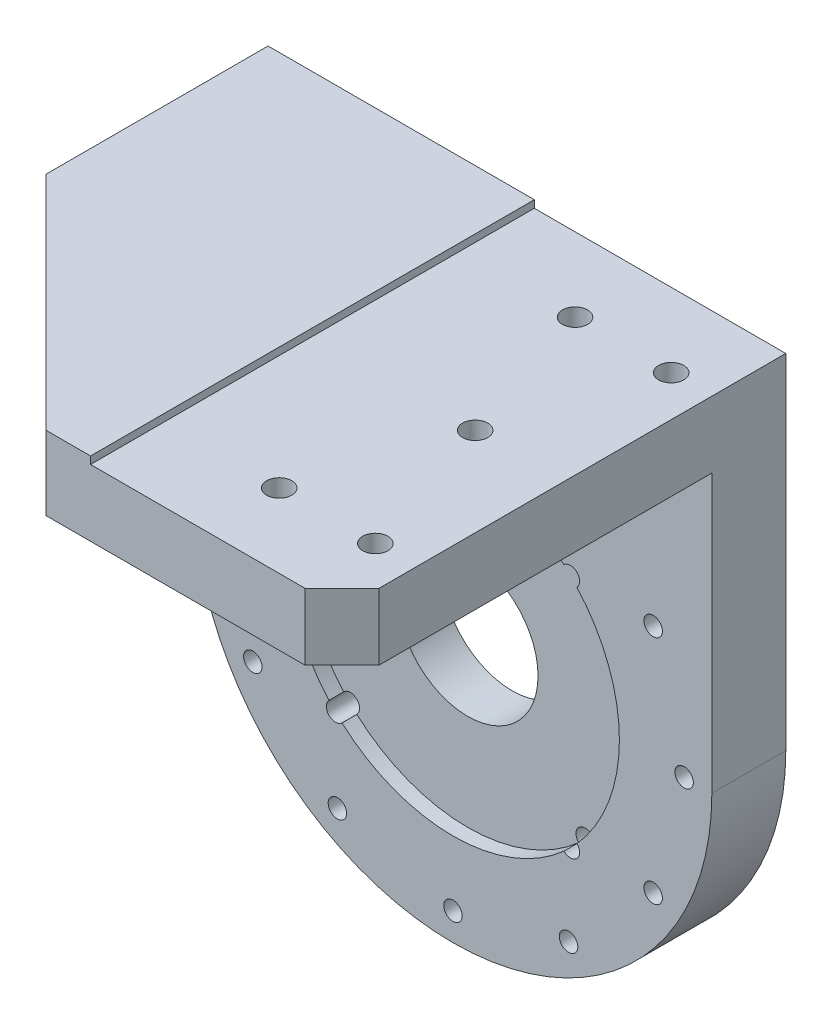
from build123d import *

# Parameters (mm, degrees)
EXTRUDE_1_DEPTH        = 20
SKETCH_2_R             = 45
CUT_EXTRUDE_1_DEPTH    = 4
SKETCH_3_R             = 19
CUT_EXTRUDE_2_DEPTH    = 104.831594421
SKETCH_4_R             = 35
CUT_EXTRUDE_3_DEPTH    = 4
HOLE_WIZARD_M6_1_D     = 5
HOLE_WIZARD_M6_2_D     = 5
SKETCH_15_W            = 140
SKETCH_15_H            = 120
EXTRUDE_2_DEPTH        = 20
SKETCH_20_W            = 68
SKETCH_20_H            = 120
CUT_EXTRUDE_4_DEPTH    = 2
CHAMFER_1_SIZE         = 10
CHAMFER_2_SIZE         = 60
HOLE_WIZARD_M8_1_D     = 6.8
HOLE_WIZARD_M8_1_DEPTH = 20


with BuildPart() as part:
    # 草图1 → 凸台-拉伸1 (new body)
    with BuildSketch(Plane.XY):
        with BuildLine():
            Line((-70, 0), (-70, 75))
            Line((-70, 75), (70, 75))
            Line((70, 75), (70, 0))
            ThreePointArc((70, 0), (0, -70), (-70, 0))
        make_face()
    extrude(amount=EXTRUDE_1_DEPTH)

    # 草图2 → 切除-拉伸1 (cut)
    with BuildSketch(Plane.XY.offset(20)):
        Circle(SKETCH_2_R)
    extrude(amount=-CUT_EXTRUDE_1_DEPTH, mode=Mode.SUBTRACT)

    # 草图3 → 切除-拉伸2 (cut, through all)
    with BuildSketch(Plane.XY.offset(16)):
        Circle(SKETCH_3_R)
    extrude(amount=-CUT_EXTRUDE_2_DEPTH, mode=Mode.SUBTRACT)

    # 草图4 → 切除-拉伸3 (cut)
    with BuildSketch(Plane(origin=(0, 0, 0), x_dir=(-1, 0, 0), z_dir=(0, 0, -1))):
        Circle(SKETCH_4_R)
    extrude(amount=-CUT_EXTRUDE_3_DEPTH, mode=Mode.SUBTRACT)

    # M6 螺纹孔1 (through all)
    with Locations(Plane.XY.offset(20)):
        with Locations((0, 62.5), (31.25, 54.126587737), (54.126587737, 31.25), (62.5, 0), (54.126587737, -31.25), (31.25, -54.126587737), (0, -62.5), (-31.25, -54.126587737), (-54.126587737, -31.25), (-62.5, 0), (-54.126587737, 31.25), (-31.25, 54.126587737)):
            Hole(HOLE_WIZARD_M6_1_D / 2)

    # M6 螺纹孔2 (through all)
    with Locations(Plane.XY.offset(20)):
        with Locations((0, 0), (31.75, 31.75), (-31.75, -31.75), (-31.75, 31.75), (31.75, -31.75)):
            Hole(HOLE_WIZARD_M6_2_D / 2)

    # 草图15 → 凸台-拉伸2 (add)
    with BuildSketch(Plane(origin=(0, 75, 0), x_dir=(1, 0, 0), z_dir=(0, 1, 0))):
        with Locations((0, -60)):
            Rectangle(SKETCH_15_W, SKETCH_15_H)
    extrude(amount=EXTRUDE_2_DEPTH)

    # 草图20 → 切除-拉伸4 (cut)
    with BuildSketch(Plane(origin=(0, 95, 0), x_dir=(1, 0, 0), z_dir=(0, 1, 0))):
        with Locations((36, -60)):
            Rectangle(SKETCH_20_W, SKETCH_20_H)
    extrude(amount=-CUT_EXTRUDE_4_DEPTH, mode=Mode.SUBTRACT)

    # 倒角1
    chamfer_1_edges = [part.edges().sort_by_distance(p)[0] for p in [
        (70, 84, 120),
    ]]
    chamfer(chamfer_1_edges, length=CHAMFER_1_SIZE)

    # 倒角2
    chamfer_2_edges = [part.edges().sort_by_distance(p)[0] for p in [
        (-70, 85, 120),
    ]]
    chamfer(chamfer_2_edges, length=CHAMFER_2_SIZE)

    # M8 螺纹孔1
    with Locations(Plane(origin=(0, 95, 0), x_dir=(1, 0, 0), z_dir=(0, 1, 0))):
        with Locations((33, -20), (59, -20), (46, -60), (33, -100), (59, -100)):
            Hole(HOLE_WIZARD_M8_1_D / 2, depth=HOLE_WIZARD_M8_1_DEPTH)


solid = part.part
